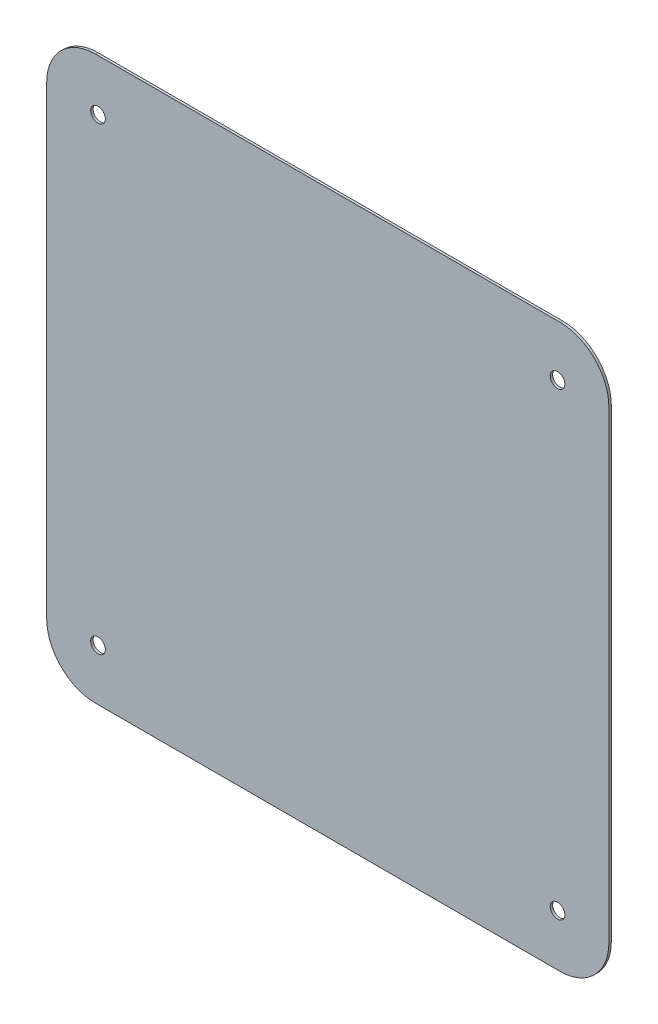
SolidWorks part; units mm, degrees
ref_plane "Front Plane" through (0, 0, 0) normal (0, 0, 1) x (1, 0, 0)
ref_plane "Top Plane" through (0, 0, 0) normal (0, 1, 0) x (1, 0, 0)
ref_plane "Right Plane" through (0, 0, 0) normal (1, 0, 0) x (0, 0, -1)
sketch "Sketch1" plane through (0, 0, 0) normal (0, 0, 1) x (1, 0, 0)
  line L1 (47.5, 57.5) -> (-47.5, 57.5)
  line L2 (57.5, 47.5) -> (57.5, -47.5)
  line L3 (47.5, -57.5) -> (-47.5, -57.5)
  line L4 (-57.5, 47.5) -> (-57.5, -47.5)
  line L5 (57.5, 57.5) -> (-57.5, -57.5) construction
  line L6 (57.5, -57.5) -> (-57.5, 57.5) construction
  line L7 (47, 47) -> (-47, 47) construction
  line L8 (47, 47) -> (47, -47) construction
  line L9 (47, -47) -> (-47, -47) construction
  line L10 (-47, 47) -> (-47, -47) construction
  line L11 (47, 47) -> (-47, -47) construction
  line L12 (47, -47) -> (-47, 47) construction
  circle A0 centre (-47, 47) radius 1.5
  circle A1 centre (47, 47) radius 1.5
  circle A2 centre (47, -47) radius 1.5
  circle A3 centre (-47, -47) radius 1.5
  arc A4 (-47.5, 57.5) -> (-57.5, 47.5) centre (-47.5, 47.5) ccw
  arc A5 (-47.5, -57.5) -> (-57.5, -47.5) centre (-47.5, -47.5) cw
  arc A6 (57.5, -47.5) -> (47.5, -57.5) centre (47.5, -47.5) cw
  arc A7 (47.5, 57.5) -> (57.5, 47.5) centre (47.5, 47.5) cw
  point P0 (0, 0)
  point P6 (0, 0)
  dimension "D5" = 3
  dimension "D6" = 10
  dimension "D1" = 115
  dimension "D2" = 115
  dimension "D3" = 94
  dimension "D4" = 94
extrude "Boss-Extrude1" add sketch "Sketch1" along normal blind 0.5
